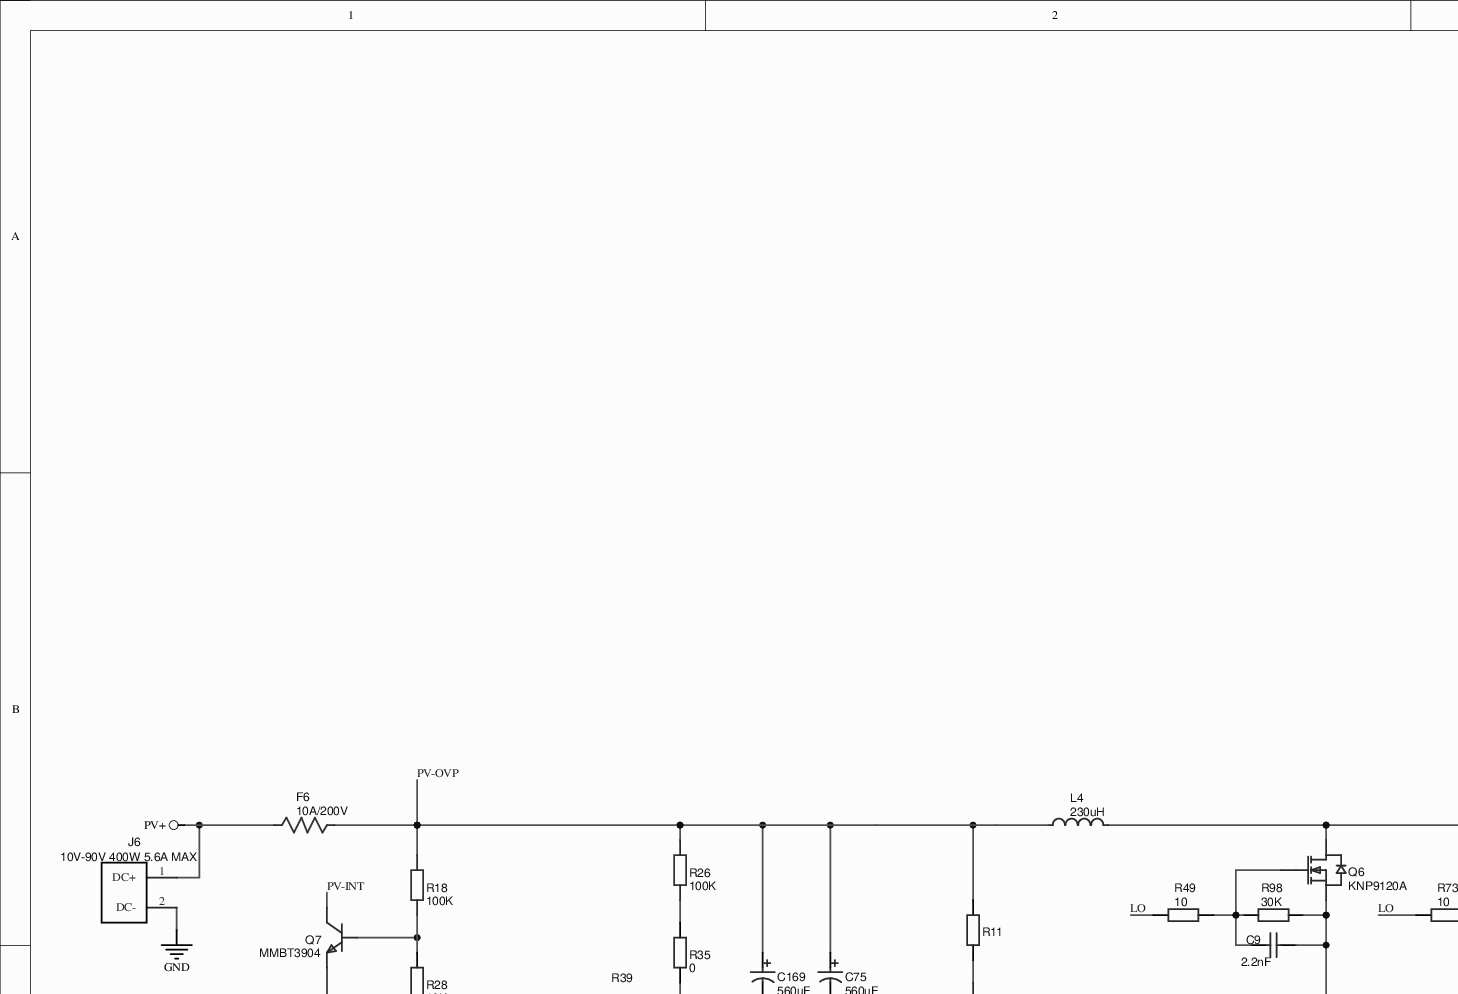
[diagram p0: MISC89356-2.schdoc, top left]
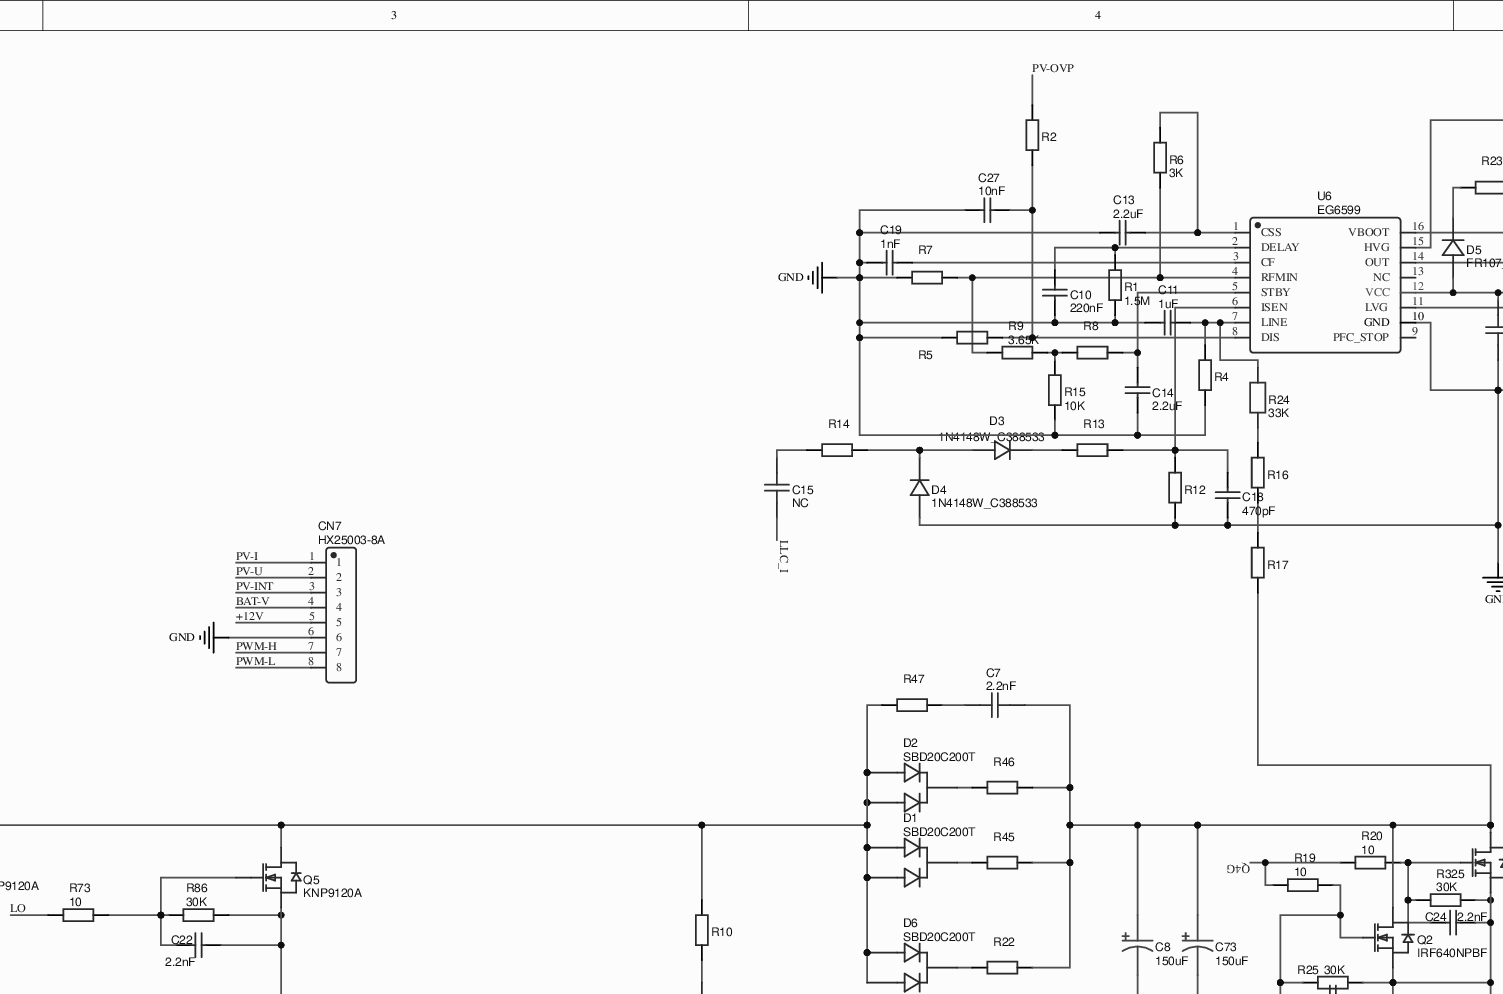
[diagram p1: MISC89356-2.schdoc, top middle]
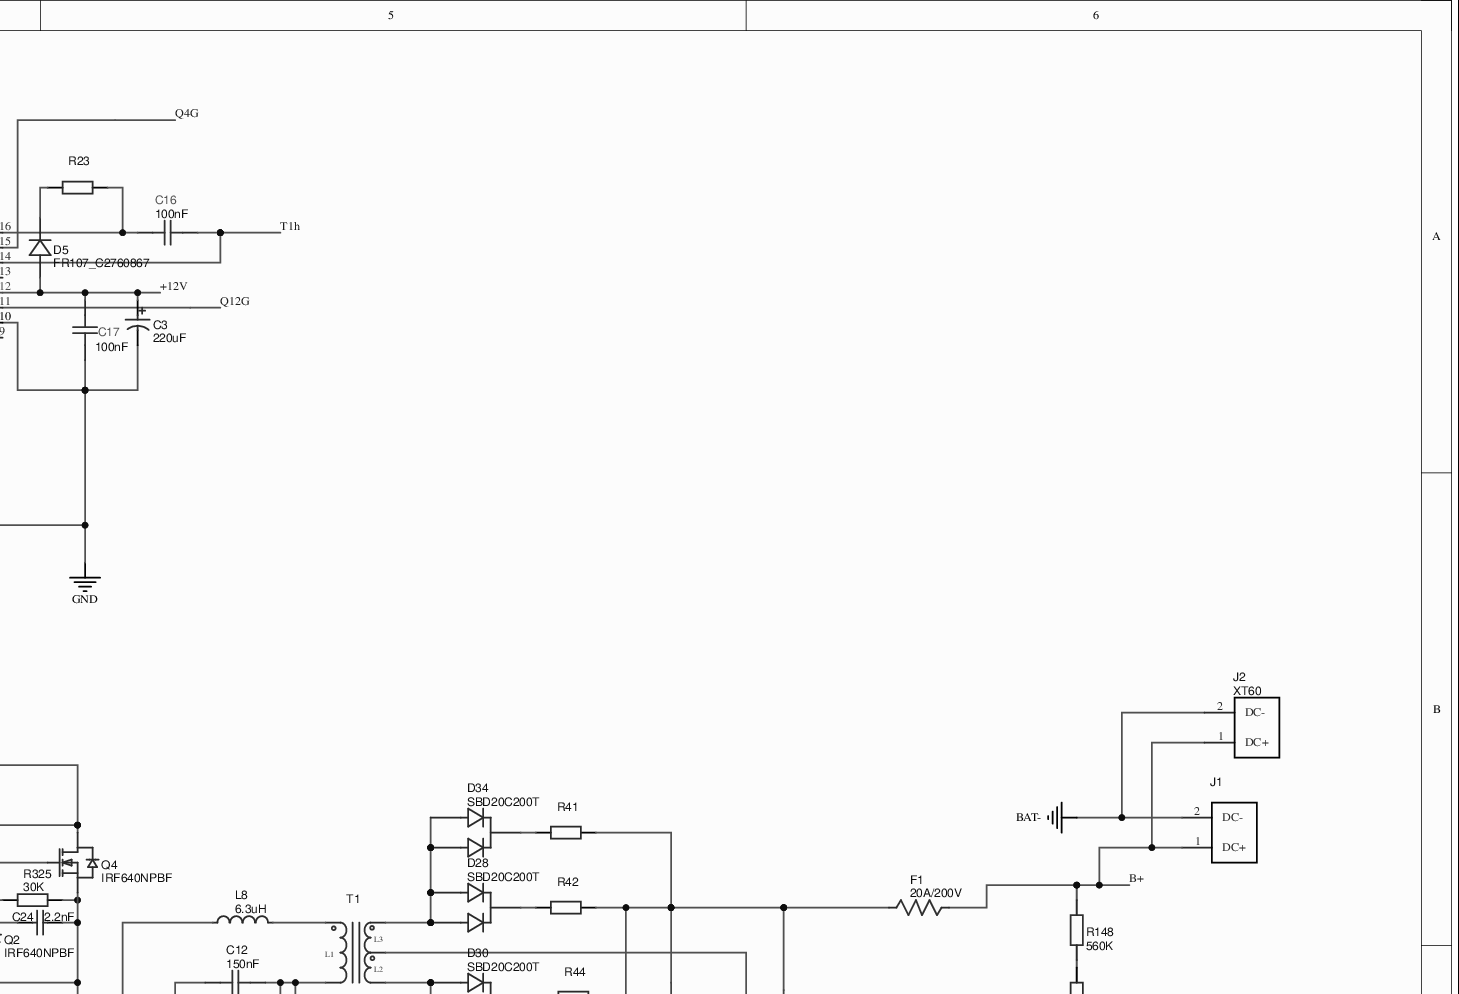
[diagram p2: MISC89356-2.schdoc, top right]
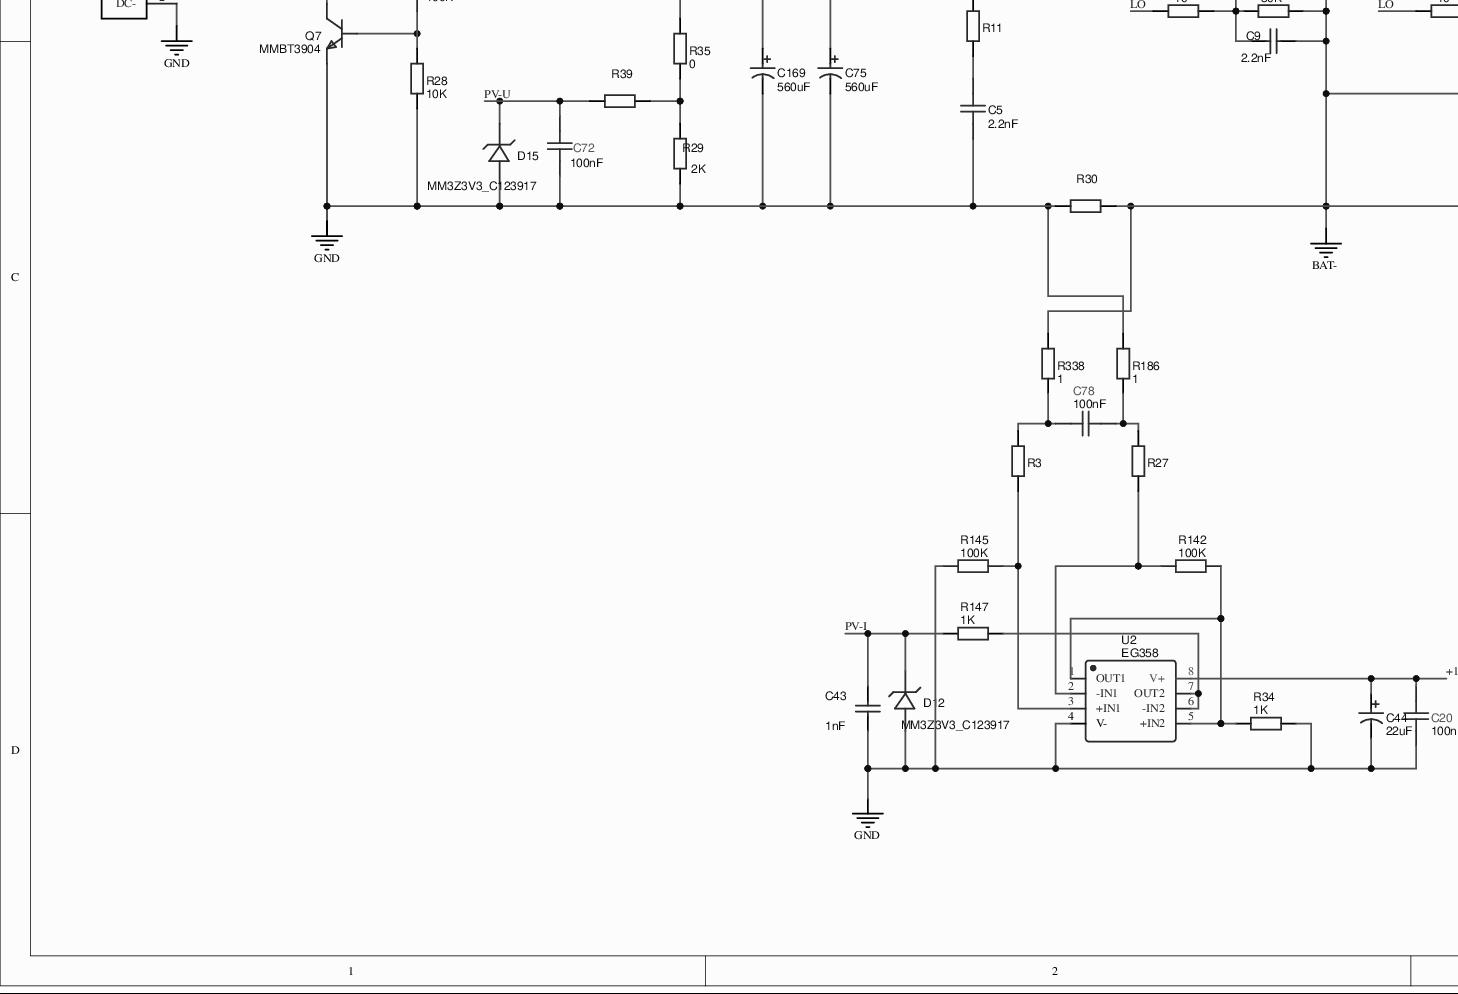
[diagram p3: MISC89356-2.schdoc, bottom left]
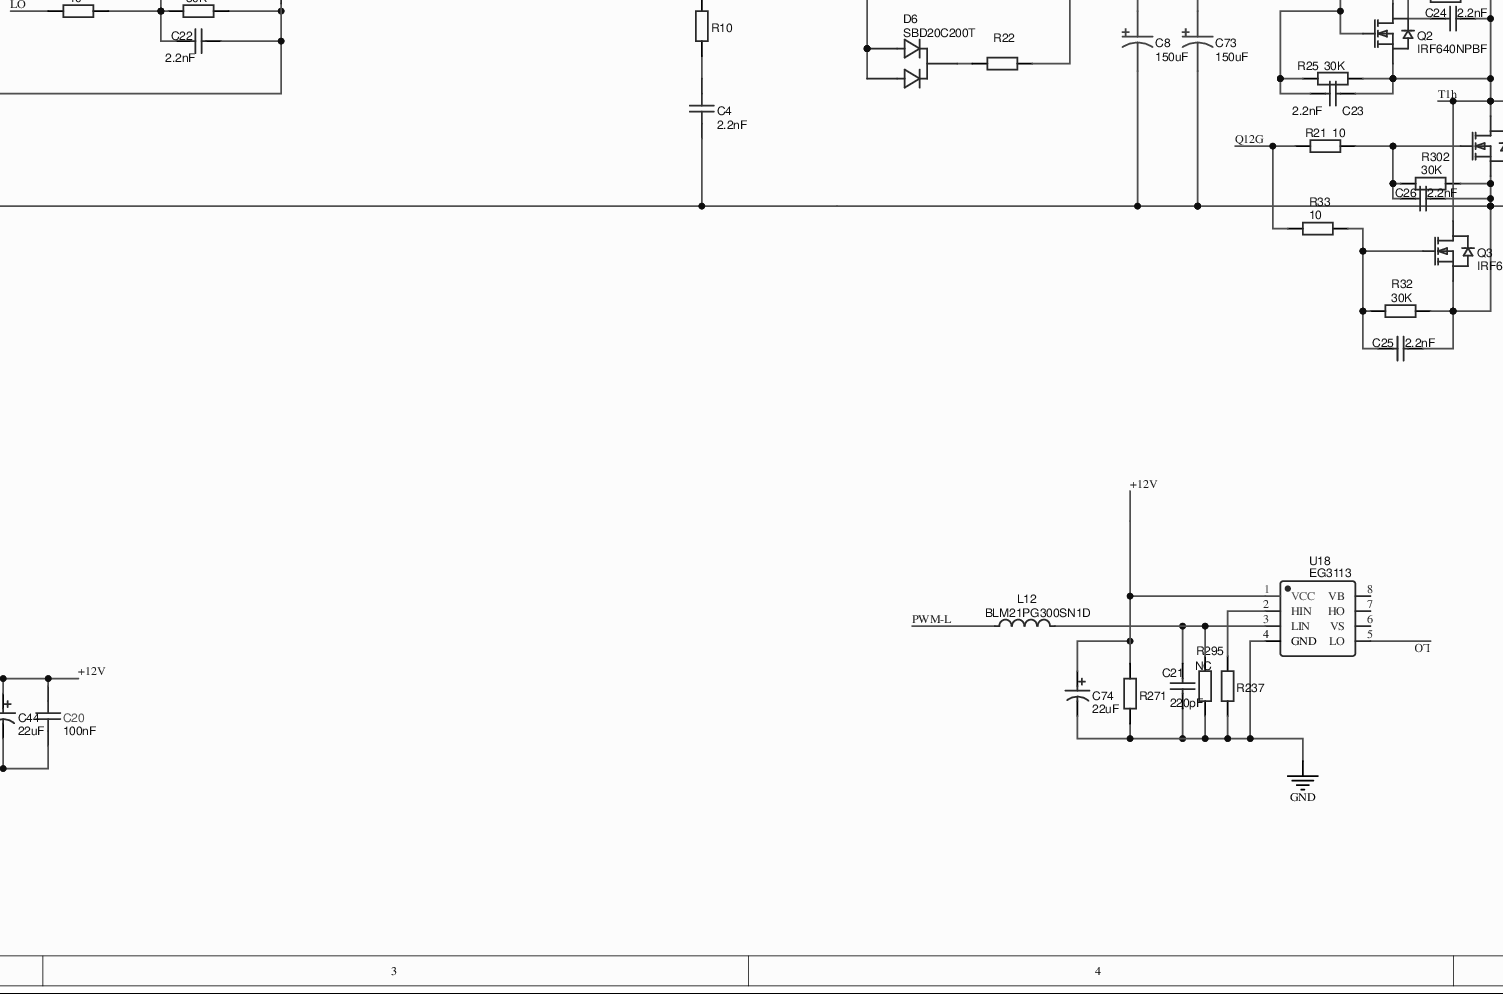
[diagram p4: MISC89356-2.schdoc, bottom middle]
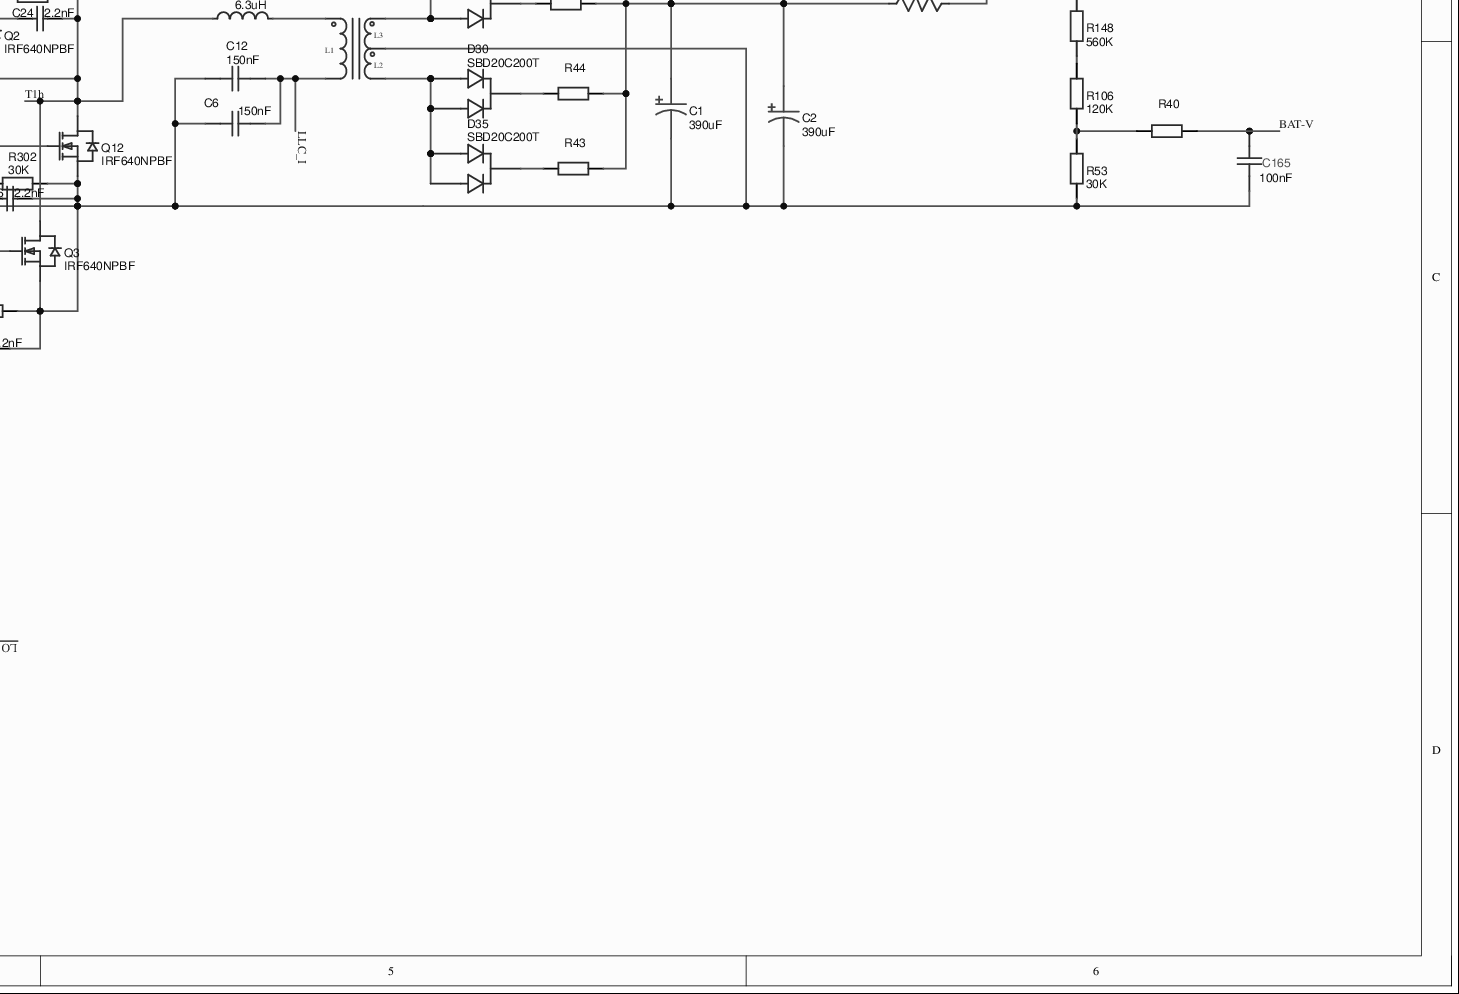
[diagram p5: MISC89356-2.schdoc, bottom right]
# Altium project MISC89356-11.PrjPCB
1 sheet, 128 parts. Net scope: global (net labels, ports and power ports of the same name join across sheets).
Board file: MISC89356.PcbDoc

## Sheet MISC89356-2.schdoc
size 715 x 319 mm

### Parts
C1  390uF  [CAP-TH_BD10.0-P5.00-D1.0-FD]
C2  390uF  [CAP-TH_BD10.0-P5.00-D1.0-FD]
C3  220uF  [CAP-TH_BD6.3-P2.50-D1.0-FD]
C4  2.2nF  [C1206]
C5  2.2nF  [C1206]
C6  150nF  [CAP-TH_L17.0-W6.5-P15.00-D1.2]
C7  2.2nF  [C1206]
C8  150uF  [CAP-TH_BD12.5-P5.00-D0.6-FD]
C9  2.2nF  [C0603]
C10  220nF  [C0603]
C11  1uF  [C0603]
C12  150nF  [CAP-TH_L17.0-W6.5-P15.00-D1.2]
C13  2.2uF  [C0603]
C14  2.2uF  [C0603]
C15  NC  [C1206]
C16  100nF  [C0603]
C17  100nF  [C0603]
C18  470pF  [C0603]
C19  1nF  [C0603]
C20  100nF  [C0603]
C21  220pF  [C0603]
C22  2.2nF  [C0603]
C23  2.2nF  [C0603]
C24  2.2nF  [C0603]
C25  2.2nF  [C0603]
C26  2.2nF  [C0603]
C27  10nF  [C1206]
C43  1nF  [C0603]
C44  22uF  [CAP-TH_BD5.0-P2.00-D0.8-FD]
C72  100nF  [C0603]
C73  150uF  [CAP-TH_BD12.5-P5.00-D0.6-FD]
C74  22uF  [CAP-TH_BD5.0-P2.00-D0.8-FD]
C75  560uF  [CAP-TH_BD16.0-P7.50-D1.2-FD]
C78  100nF  [C0603]
C165  100nF  [C0603]
C169  560uF  [CAP-TH_BD16.0-P7.50-D1.2-FD]
CN7  HX25003-8A  [CONN-TH_8P-P2.50_HX25003-8A]
D1  SBD20C200T  [TO-220-3_L10.0-W4.5-P2.54-L]
D2  SBD20C200T  [TO-220-3_L10.0-W4.5-P2.54-L]
D3  1N4148W_C388533  [SOD-123_L2.8-W1.8-LS3.7-RD]
D4  1N4148W_C388533  [SOD-123_L2.8-W1.8-LS3.7-RD]
D5  FR107_C2760867  [SOD-123FL_L2.7-W1.8-LS3.8-RD]
D6  SBD20C200T  [TO-220-3_L10.0-W4.5-P2.54-L]
D12  MM3Z3V3_C123917  [SOD-323_L1.8-W1.3-LS2.5-RD]
D15  MM3Z3V3_C123917  [SOD-323_L1.8-W1.3-LS2.5-RD]
D28  SBD20C200T  [TO-220-3_L10.0-W4.5-P2.54-L-N]
D30  SBD20C200T  [TO-220-3_L10.0-W4.5-P2.54-L-N]
D34  SBD20C200T  [TO-220-3_L10.0-W4.5-P2.54-L-N]
D35  SBD20C200T  [TO-220-3_L10.0-W4.5-P2.54-L-N]
F1  20A/200V  [FUSE-SMD_L6.1-W2.5]
F6  10A/200V  [FUSE-SMD_L6.1-W2.5]
J1  (no value)  [XT90N]
J2  XT60  [CONN-TH_XT60UPB-F]
J6  10V-90V 400W 5.6A MAX  [XT90]
L4  230uH  [IND-TH_CS343090*2-W231K]
L8  6.3uH  [PQ2620-N]
L12  BLM21PG300SN1D  [L0805]
Q2  IRF640NPBF  [TO-220-3_L10.0-W4.5-P2.54-L-N]
Q3  IRF640NPBF  [TO-220-3_L10.0-W4.5-P2.54-L-N]
Q4  IRF640NPBF  [TO-220-3_L10.0-W4.5-P2.54-L-N]
Q5  KNP9120A  [TO-220-3_L10.0-W4.5-P2.54-L]
Q6  KNP9120A  [TO-220-3_L10.0-W4.5-P2.54-L]
Q7  MMBT3904  [SOT-23-3_L2.9-W1.3-P1.90-LS2.4-BR]
Q12  IRF640NPBF  [TO-220-3_L10.0-W4.5-P2.54-L-N]
R1  1.5M  [R0603]
R2  (no value)  [R0805]
R3  (no value)  [R0603]
R4  (no value)  [R0603]
R5  (no value)  [R0805]
R6  3K  [R0603]
R7  (no value)  [R0603]
R8  (no value)  [R0603]
R9  3.65K  [R0603]
R10  (no value)  [R1206]
R11  (no value)  [R1206]
R12  (no value)  [R0603]
R13  (no value)  [R0603]
R14  (no value)  [R0603]
R15  10K  [R1206]
R16  (no value)  [R1206]
R17  (no value)  [R1206]
R18  100K  [R0805]
R19  10  [R1206]
R20  10  [R1206]
R21  10  [R1206]
R22  (no value)  [R2512]
R23  (no value)  [R0805]
R24  33K  [R1206]
R25  30K  [R0603]
R26  100K  [R0805]
R27  (no value)  [R0603]
R28  10K  [R1206]
R29  2K  [R0603]
R30  (no value)  [R2512]
R32  30K  [R0603]
R33  10  [R1206]
R34  1K  [R0603]
R35  0  [R0805]
R39  (no value)  [R0603]
R40  (no value)  [R0603]
R41  (no value)  [R2512]
R42  (no value)  [R2512]
R43  (no value)  [R2512]
R44  (no value)  [R2512]
R45  (no value)  [R2512]
R46  (no value)  [R2512]
R47  (no value)  [R1206]
R49  10  [R1206]
R53  30K  [R0603]
R73  10  [R1206]
R86  30K  [R0603]
R98  30K  [R0603]
R106  120K  [R0603]
R142  100K  [R0805]
R145  100K  [R0805]
R147  1K  [R0603]
R148  560K  [R0603]
R186  1  [R0603]
R237  (no value)  [R0603]
R271  (no value)  [R0603]
R295  NC  [R0603]
R302  30K  [R0603]
R325  30K  [R0603]
R338  1  [R0603]
T1  (no value)  [PQ3230 3:2:2-N]
U2  EG358  [SOIC-8_L5.0-W4.0-P1.27-LS6.0-BL]
U6  EG6599  [SO-16_L10.0-W4.0-P1.27-LS6.2-BL]
U18  EG3113  [SOP-8_L4.9-W3.9-P1.27-LS6.0-BL]

### Nets
BAT-: C1.2 C2.2 C4.2 C6.2 C8.2 C9.2 C12.2 C22.2 C25.2 C26.2 C73.2 C165.1 J1.2(DC-) J2.2(DC-) Q3.3(S) Q5.3(S) Q6.3(S) Q12.3(S) R30.2 R32.2 R53.1 R86.1 R98.1 R302.2 R338.2 T1.9
GND: C3.2 C5.2 C10.1 C11.2 C13.1 C14.1 C17.1 C18.1 C19.2 C20.2 C21.1 C27.1 C43.1 C44.2 C72.1 C74.2 C75.2 C169.2 CN7.6 D4.2(A) D12.2(A) D15.2(A) J6.2(DC-) Q7.2(E) R1.1 R4.1 R5.1 R7.2 R12.1 R15.2 R28.2 R29.2 R30.1 R34.2 R145.2 R186.2 R237.1 R271.1 R295.2 U2.4(V-) U6.10(GND) U18.4(GND)
PV+: F6.1 J6.1(DC+)
+12V: C3.1 C17.2 C20.1 C44.1 C74.1 CN7.5 D5.2(A) R271.2 U2.8(V+) U6.12(VCC) U18.1(VCC)
B+: F1.2 J1.1(DC+) J2.1(DC+) R148.2
BAT-V: C165.2 CN7.4 R40.1
LLC_I: C6.1 C12.1 C15.1 T1.3
LO: R49.1 R73.1 U18.5(LO)
PV-I: C43.2 CN7.1 D12.1(K) R147.2
PV-INT: CN7.3 Q7.3(C)
PV-OVP: C75.1 C169.1 F6.2 L4.1 R2.2 R11.1 R18.2 R26.2
PV-U: C72.2 CN7.2 D15.1(K) R39.2
PWM-H: CN7.7
PWM-L: CN7.8 L12.1
Q4G: R19.1 R20.1 U6.15(HVG)
Q12G: R21.1 R33.1 U6.11(LVG)
T1h: C16.1 C23.2 C24.2 L8.3 Q2.3(S) Q3.2(D) Q4.3(S) Q12.2(D) R25.2 R325.2 U6.14(OUT)
NetC1_1: C1.1 C2.1 F1.1 R41.2 R42.2 R43.2 R44.2
NetC4_1: C4.1 R10.2
NetC5_1: C5.1 R11.2
NetC7_1: C7.1 R47.2
NetC7_2: C7.2 C8.1 C73.1 Q2.2(D) Q4.2(D) R17.1 R22.2 R45.2 R46.2
NetC9_1: C9.1 Q6.1(G) R49.2 R98.2
NetC10_2: C10.2 R1.2 U6.2(DELAY)
NetC11_1: C11.1 R4.2 R24.2 U6.7(LINE)
NetC13_2: C13.2 R6.2 U6.1(CSS)
NetC14_2: C14.2 R8.2 U6.5(STBY)
NetC15_2: C15.2 R14.1
NetC16_2: C16.2 R23.1 U6.16(VBOOT)
NetC18_2: C18.2 R12.2 R13.2 U6.6(ISEN)
NetC19_1: C19.1 U6.3(CF)
NetC21_2: C21.2 L12.2 R295.1 U18.3(LIN)
NetC22_1: C22.1 Q5.1(G) R73.2 R86.2
NetC23_1: C23.1 Q2.1(G) R19.2 R25.1
NetC24_1: C24.1 Q4.1(G) R20.2 R325.1
NetC25_1: C25.1 Q3.1(G) R32.1 R33.2
NetC26_1: C26.1 Q12.1(G) R21.2 R302.1
NetC27_2: C27.2 R2.1 R5.2 U6.8(DIS)
NetC78_1: C78.1 R27.2 R186.1
NetC78_2: C78.2 R3.2 R338.1
NetD1_1: D1.1 D1.3 D2.1 D2.3 D6.1 D6.3 L4.2 Q5.2(D) Q6.2(D) R10.1 R47.1
NetD1_2: D1.2 R45.1
NetD2_2: D2.2 R46.1
NetD3_1: D3.1(C) R13.1
NetD3_2: D3.2(A) D4.1(C) R14.2
NetD5_1: D5.1(K) R23.2
NetD6_2: D6.2 R22.1
NetD28_1: D28.1 D28.3 D34.1 D34.3 T1.8
NetD28_2: D28.2 R42.1
NetD30_1: D30.1 D30.3 D35.1 D35.3 T1.10
NetD30_2: D30.2 R44.1
NetD34_2: D34.2 R41.1
NetD35_2: D35.2 R43.1
NetL8_4: L8.4 T1.4
NetQ7_1: Q7.1(B) R18.1 R28.1
NetR3_1: R3.1 R145.1 U2.3(+IN1)
NetR6_1: R6.1 R7.1 R9.1 U6.4(RFMIN)
NetR8_1: R8.1 R9.2 R15.1
NetR16_1: R16.1 R17.2
NetR16_2: R16.2 R24.1
NetR26_1: R26.1 R35.2
NetR27_1: R27.1 R142.2 U2.2(-IN1)
NetR29_1: R29.1 R35.1 R39.1
NetR34_1: R34.1 R142.1 U2.1(OUT1) U2.5(+IN2)
NetR40_2: R40.2 R53.2 R106.1
NetR106_2: R106.2 R148.1
NetR147_1: R147.1 U2.6(-IN2) U2.7(OUT2)
NetR237_2: R237.2 U18.2(HIN)

Not connected (* = marked no-connect by the designer): U6 9(PFC_STOP) 13(NC); U18 6(VS) 7(HO) 8(VB)

### Library data of the parts
C1 C2 = 390uF: BOM_Manufacturer: Ymin; BOM_Manufacturer Part: LKME2001J391MF; nameAlias: Capacitance; Contributor: LCSC; BOM_Supplier: LCSC; BOM_Supplier Part: C442948; BOM_JLCPCB Part Class: Extended Part; spicePre: C; spiceSymbolName: LKME2001J391MF
C3 = 220uF: BOM_Manufacturer: ValuePro; BOM_Manufacturer Part: 220uF 16V 6.3*11; nameAlias: Capacitance; BOM_Supplier: LCSC; BOM_Supplier Part: C43349; BOM_JLCPCB Part Class: Extended Part; spicePre: C; spiceSymbolName: 220uF 16V 6.3*11
C4 C5 C7 = 2.2nF: BOM_Manufacturer: Johanson Dielectrics; BOM_Manufacturer Part: 202R18W222KV4E; nameAlias: Capacitance; Contributor: LCSC; BOM_Supplier: LCSC; BOM_Supplier Part: C173213; BOM_JLCPCB Part Class: Extended Part; spicePre: C; spiceSymbolName: 202R18W222KV4E
C6 C12 = 150nF: BOM_Manufacturer: KYET; BOM_Manufacturer Part: KP154J2J1501; nameAlias: Capacitance; Contributor: LCSC; BOM_Supplier: LCSC; BOM_Supplier Part: C390138; BOM_JLCPCB Part Class: Extended Part; spicePre: C; spiceSymbolName: KP154J2J1501
C8 C73 = 150uF: BOM_Manufacturer: Ymin; BOM_Manufacturer Part: LKML2502C151MF; nameAlias: Capacitance; Contributor: LCSC; BOM_Supplier: LCSC; BOM_Supplier Part: C443216; BOM_JLCPCB Part Class: Extended Part; spicePre: C; spiceSymbolName: LKML2502C151MF
C9 C22-C26 = 2.2nF: BOM_Manufacturer: YAGEO; BOM_Manufacturer Part: CC0603KRX7R9BB222; nameAlias: Capacitance; BOM_Supplier: LCSC; BOM_Supplier Part: C107082; BOM_JLCPCB Part Class: Extended Part; spicePre: C; spiceSymbolName: CC0603KRX7R9BB222
C10 = 220nF: BOM_Manufacturer Part: CL10B224KA8NNNC; BOM_Manufacturer: SAMSUNG; nameAlias: Capacitance; BOM_Supplier: LCSC; BOM_Supplier Part: C21120; BOM_JLCPCB Part Class: Basic Part; spicePre: C; spiceSymbolName: CL10B224KA8NNNC
C11 = 1uF: BOM_Manufacturer Part: CL10A105KB8NNNC; BOM_Manufacturer: SAMSUNG; nameAlias: Capacitance; BOM_Supplier: LCSC; BOM_Supplier Part: C15849; BOM_JLCPCB Part Class: Basic Part; spicePre: C; spiceSymbolName: CL10A105KB8NNNC
C13 C14 = 2.2uF: BOM_Manufacturer Part: CL10A225KO8NNNC; BOM_Manufacturer: SAMSUNG; nameAlias: Capacitance; BOM_Supplier: LCSC; BOM_Supplier Part: C23630; BOM_JLCPCB Part Class: Basic Part; spicePre: C; spiceSymbolName: CL10A225KO8NNNC
C15 = NC: BOM_Manufacturer: Guangdong Fenghua Advanced Tech; BOM_Manufacturer Part: 1206CG220J102NT; nameAlias: Capacitance; Contributor: LCSC; BOM_Supplier: LCSC; BOM_Supplier Part: C313096; BOM_JLCPCB Part Class: Extended Part; spicePre: C; spiceSymbolName: 1206CG220J102NT
C16 C17 C20 C72 C78 C165 = 100nF: BOM_Manufacturer: SAMSUNG; BOM_Manufacturer Part: CL10B104KC8NNNC; nameAlias: Capacitance; BOM_Supplier: LCSC; BOM_Supplier Part: C15725; BOM_JLCPCB Part Class: Extended Part; spicePre: C; spiceSymbolName: CL10B104KC8NNNC
C18 = 470pF: BOM_Manufacturer: FH; BOM_Manufacturer Part: 0603B471K500NT; nameAlias: Capacitance; BOM_Supplier: LCSC; BOM_Supplier Part: C1620; BOM_JLCPCB Part Class: Basic Part; spicePre: C; spiceSymbolName: 0603B471K500NT
C19 = 1nF: BOM_Manufacturer: SAMSUNG; BOM_Manufacturer Part: CL10B102KB8NNNC; nameAlias: Capacitance; Contributor: LCSC; BOM_Supplier: LCSC; BOM_Supplier Part: C1588; BOM_JLCPCB Part Class: Extended Part; spicePre: C; spiceSymbolName: CL10B102KC8NNNC
C21 = 220pF: BOM_Manufacturer: YAGEO; BOM_Manufacturer Part: CC0603KRX7R9BB221; nameAlias: Capacitance; BOM_Supplier: LCSC; BOM_Supplier Part: C107081; BOM_JLCPCB Part Class: Extended Part; spicePre: C; spiceSymbolName: CC0603KRX7R9BB221
C27 = 10nF: BOM_Manufacturer: FH; BOM_Manufacturer Part: 1206B103K102NT; nameAlias: Capacitance; BOM_Supplier: LCSC; BOM_Supplier Part: C9194; BOM_JLCPCB Part Class: Extended Part; spicePre: C; spiceSymbolName: 1206B103K102NT
C43 = 1nF: BOM_Manufacturer Part: CL10B102KB8NNNC; BOM_Manufacturer: SAMSUNG; nameAlias: Capacitance; BOM_Supplier: LCSC; BOM_Supplier Part: C1588; BOM_JLCPCB Part Class: Basic Part; spicePre: C; spiceSymbolName: CL10B102KB8NNNC
C44 C74 = 22uF: BOM_Manufacturer: ValuePro; BOM_Manufacturer Part: 22uF 50V 5*11; nameAlias: Capacitance; BOM_Supplier: LCSC; BOM_Supplier Part: C43346; BOM_JLCPCB Part Class: Extended Part; spicePre: C; spiceSymbolName: 22uF 50V 5*11
C75 C169 = 560uF: BOM_Manufacturer: Rubycon; BOM_Manufacturer Part: 35YXJ2200M16X25; nameAlias: Capacitance; BOM_Supplier: LCSC; BOM_Supplier Part: C95096; BOM_JLCPCB Part Class: Extended Part; spicePre: C; spiceSymbolName: 35YXJ2200M16X25
CN7 = HX25003-8A: BOM_Manufacturer: HX(Zhejiang Yueqing Hongxing Elec); Contributor: LCSC; BOM_Supplier: LCSC; BOM_Supplier Part: C442305; BOM_Manufacturer Part: HX25003-8A; BOM_JLCPCB Part Class: Extended Part; spicePre: C; spiceSymbolName: HX25003-8A
D1 D2 D6 D28 D30 D34 D35 = SBD20C200T: BOM_Manufacturer: PANJIT; BOM_Manufacturer Part: SBT40100VCT; Contributor: LCSC; BOM_Supplier Part: C142331; BOM_Supplier: LCSC; BOM_JLCPCB Part Class: Extended Part; spicePre: D; spiceSymbolName: SBT40100VCT
D3 D4 = 1N4148W_C388533: BOM_Manufacturer: Yangzhou Yangjie Elec Tech; Contributor: LCSC; BOM_Supplier: LCSC; BOM_Supplier Part: C388533; BOM_Manufacturer Part: 1N4148W; BOM_JLCPCB Part Class: Extended Part; spicePre: D; spiceSymbolName: 1N4148W_C388533
D5 = FR107_C2760867: BOM_Manufacturer Part: FR107; Contributor: LCSC; BOM_Supplier: LCSC; BOM_Supplier Part: C2760867; BOM_JLCPCB Part Class: Extended Part; spicePre: D; spiceSymbolName: FR107_C2760867
D12 D15 = MM3Z3V3_C123917: BOM_Manufacturer: Shandong Jingdao Microelectronics; Contributor: LCSC; BOM_Supplier: LCSC; BOM_Supplier Part: C123917; BOM_Manufacturer Part: MM3Z3V3; BOM_JLCPCB Part Class: Extended Part; spicePre: D; spiceSymbolName: MM3Z3V3_C123917
F1 = 20A/200V: Contributor: LCEDA_Lib; spicePre: R; spiceSymbolName: R_1206_US
F6 = 10A/200V: Contributor: LCEDA_Lib; spicePre: R; spiceSymbolName: R_1206_US
J1 = (no symbol name): BOM_Manufacturer: ReliaPro; BOM_Manufacturer Part: TJC1-2A; BOM_Supplier: LCSC; BOM_Supplier Part: C29632; spicePre: J; spiceSymbolName: TJC1-2A
J2 = XT60: BOM_Manufacturer: ReliaPro; BOM_Manufacturer Part: TJC1-2A; BOM_Supplier: LCSC; BOM_Supplier Part: C29632; spicePre: J; spiceSymbolName: TJC1-2A
J6 = 10V-90V 400W 5.6A MAX: BOM_Manufacturer: ReliaPro; BOM_Manufacturer Part: TJC1-2A; BOM_Supplier: LCSC; BOM_Supplier Part: C29632; spicePre: J; spiceSymbolName: TJC1-2A
L4 = 230uH: nameAlias: Value(H); Contributor: LCEDA_Lib; spicePre: L; spiceSymbolName: L0402_US
L8 = 6.3uH: nameAlias: Value(H); Contributor: LCEDA_Lib; spicePre: L; spiceSymbolName: L0402_US
L12 = BLM21PG300SN1D: BOM_Manufacturer: MuRata; nameAlias: Value(H); BOM_Supplier: LCSC; BOM_Manufacturer Part: BLM21PG300SN1D; BOM_Supplier Part: C16903; BOM_JLCPCB Part Class: Extended Part; spicePre: L; spiceSymbolName: BLM21PG300SN1D
Q2-Q4 Q12 = IRF640NPBF: BOM_Manufacturer: Infineon; BOM_Supplier: LCSC; BOM_Manufacturer Part: IRF640NPBF; BOM_Supplier Part: C2568; BOM_JLCPCB Part Class: Extended Part; spicePre: Q; spiceSymbolName: IRF640NPBF
Q5 Q6 = KNP9120A: BOM_Manufacturer: KIA; BOM_Supplier: LCSC; BOM_Manufacturer Part: KNP9120A; BOM_Supplier Part: C135565; BOM_JLCPCB Part Class: Extended Part; spicePre: Q; spiceSymbolName: KNP9120A
Q7 = MMBT3904: Contributor: LCSC; BOM_Supplier: LCSC; BOM_Supplier Part: C2688228; BOM_Manufacturer Part: MMBT3904; BOM_JLCPCB Part Class: Extended Part; spicePre: Q; spiceSymbolName: MMBT3904
R1 = 1.5M: BOM_Manufacturer: YAGEO; BOM_Manufacturer Part: RC0603FR-071M5L; nameAlias: Resistance (Ohms); BOM_Supplier: LCSC; BOM_Supplier Part: C137773; BOM_JLCPCB Part Class: Extended Part; spicePre: R; spiceSymbolName: RC0603FR-071M5L
R2 = (no symbol name): BOM_Manufacturer: UniOhm; BOM_Manufacturer Part: 0805W8F4753T5E; nameAlias: Resistance; Resistance (Ohms): 475K; BOM_Supplier: LCSC; BOM_Supplier Part: C17711; BOM_JLCPCB Part Class: Extended Part; spicePre: R; spiceSymbolName: 0805W8F4753T5E
R3 R12 R27 = (no symbol name): BOM_Manufacturer: UniOhm; BOM_Manufacturer Part: 0603WAF1501T5E; nameAlias: Resistance; Resistance (Ohms): 1.5K; BOM_Supplier: LCSC; BOM_Supplier Part: C22843; BOM_JLCPCB Part Class: Basic Part; spicePre: R; spiceSymbolName: 0603WAF1501T5E
R4 R14 R271 = (no symbol name): BOM_Manufacturer: UniOhm; BOM_Manufacturer Part: 0603WAF1002T5E; nameAlias: Resistance; Resistance (Ohms): 10K; BOM_Supplier: LCSC; BOM_Supplier Part: C25804; BOM_JLCPCB Part Class: Basic Part; spicePre: R; spiceSymbolName: 0603WAF1002T5E
R5 = (no symbol name): BOM_Manufacturer: UniOhm; BOM_Manufacturer Part: 0805W8F9101T5E; nameAlias: Resistance; Resistance (Ohms): 9.1K; BOM_Supplier: LCSC; BOM_Supplier Part: C17855; BOM_JLCPCB Part Class: Basic Part; spicePre: R; spiceSymbolName: 0805W8F9101T5E
R6 = 3K: BOM_Manufacturer: YAGEO; BOM_Manufacturer Part: RC0603FR-073KL; nameAlias: Resistance (Ohms); BOM_Supplier: LCSC; BOM_Supplier Part: C126358; BOM_JLCPCB Part Class: Extended Part; spicePre: R; spiceSymbolName: RC0603FR-073KL
R7 = (no symbol name): BOM_Manufacturer: UniOhm; BOM_Manufacturer Part: 0603WAF4701T5E; nameAlias: Resistance; Resistance (Ohms): 4.7K; BOM_Supplier: LCSC; BOM_Supplier Part: C23162; BOM_JLCPCB Part Class: Basic Part; spicePre: R; spiceSymbolName: 0603WAF4701T5E
R8 R237 = (no symbol name): BOM_Manufacturer: UniOhm; BOM_Manufacturer Part: 0603WAF0000T5E; nameAlias: Resistance; Resistance (Ohms): 0; BOM_Supplier: LCSC; BOM_Supplier Part: C21189; BOM_JLCPCB Part Class: Basic Part; spicePre: R; spiceSymbolName: 0603WAF0000T5E
R9 = 3.65K: BOM_Manufacturer: YAGEO; BOM_Manufacturer Part: RC0603FR-073K65L; nameAlias: Resistance (Ohms); BOM_Supplier: LCSC; BOM_Supplier Part: C137730; BOM_JLCPCB Part Class: Extended Part; spicePre: R; spiceSymbolName: RC0603FR-073K65L
R10 R11 R47 = (no symbol name): BOM_Manufacturer: UniOhm; BOM_Manufacturer Part: 1206W4F100KT5E; nameAlias: Resistance; Resistance (Ohms): 1; BOM_Supplier: LCSC; BOM_Supplier Part: C17928; BOM_JLCPCB Part Class: Basic Part; spicePre: R; spiceSymbolName: 1206W4F100KT5E
R13 = (no symbol name): BOM_Manufacturer: UniOhm; BOM_Manufacturer Part: 0603WAF510JT5E; nameAlias: Resistance; Resistance (Ohms): 51; BOM_Supplier: LCSC; BOM_Supplier Part: C23197; BOM_JLCPCB Part Class: Basic Part; spicePre: R; spiceSymbolName: 0603WAF510JT5E
R15 R28 = 10K: BOM_Manufacturer: UniOhm; BOM_Manufacturer Part: 1206W4F1002T5E; nameAlias: Resistance (Ohms); BOM_Supplier: LCSC; BOM_Supplier Part: C17902; BOM_JLCPCB Part Class: Basic Part; spicePre: R; spiceSymbolName: 1206W4F1002T5E
R16 R17 = (no symbol name): BOM_Manufacturer: UniOhm; BOM_Manufacturer Part: 1206W4F3003T5E; nameAlias: Resistance; Resistance (Ohms): 300K; BOM_Supplier: LCSC; BOM_Supplier Part: C17884; BOM_JLCPCB Part Class: Extended Part; spicePre: R; spiceSymbolName: 1206W4F3003T5E
R18 R26 R142 R145 = 100K: BOM_Manufacturer: YAGEO; BOM_Manufacturer Part: RC0805JR-07100KL; nameAlias: Resistance (Ohms); Contributor: LCSC; BOM_Supplier: LCSC; BOM_Supplier Part: C100049; BOM_JLCPCB Part Class: Extended Part; spicePre: R; spiceSymbolName: RC0805JR-07100KL
R19-R21 R33 R49 R73 = 10: BOM_Manufacturer: LIZ; BOM_Manufacturer Part: CR1206J40100G; nameAlias: Resistance (Ohms); BOM_Supplier: LCSC; BOM_Supplier Part: C102266; BOM_JLCPCB Part Class: Extended Part; spicePre: R; spiceSymbolName: CR1206J40100G
R22 R41-R46 = (no symbol name): BOM_Manufacturer: RALEC; BOM_Manufacturer Part: RTT25R100FTE; nameAlias: Resistance; Resistance (Ohms): 0.1; BOM_Supplier: LCSC; BOM_Supplier Part: C105145; BOM_JLCPCB Part Class: Extended Part; spicePre: R; spiceSymbolName: RTT25R100FTE
R23 = (no symbol name): BOM_Manufacturer: UniOhm; BOM_Manufacturer Part: 0805W8F220KT5E; nameAlias: Resistance; Resistance (Ohms): 2.2; BOM_Supplier: LCSC; BOM_Supplier Part: C17521; BOM_JLCPCB Part Class: Basic Part; spicePre: R; spiceSymbolName: 0805W8F220KT5E
R24 = 33K: BOM_Manufacturer: YAGEO; BOM_Manufacturer Part: AC1206JR-0733KL; nameAlias: Resistance (Ohms); Contributor: LCSC; BOM_Supplier: LCSC; BOM_Supplier Part: C229931; BOM_JLCPCB Part Class: Extended Part; spicePre: R; spiceSymbolName: AC1206JR-0733KL
R25 R32 R53 R86 R98 R302 R325 = 30K: BOM_Manufacturer: UniOhm; BOM_Manufacturer Part: 0805W8F3002T5E; nameAlias: Resistance (Ohms); BOM_Supplier: LCSC; BOM_Supplier Part: C17621; BOM_JLCPCB Part Class: Basic Part; spicePre: R; spiceSymbolName: 0805W8F3002T5E
R29 = 2K: BOM_Manufacturer: UniOhm; BOM_Manufacturer Part: 0603WAF2001T5E; nameAlias: Resistance (Ohms); BOM_Supplier: LCSC; BOM_Supplier Part: C22975; BOM_JLCPCB Part Class: Basic Part; spicePre: R; spiceSymbolName: 0603WAF2001T5E
R30 = (no symbol name): BOM_Manufacturer: PSA; BOM_Manufacturer Part: FMF25FPHR005-LHL; nameAlias: Resistance; Resistance (Ohms): 0.005; BOM_Supplier: LCSC; BOM_Supplier Part: C105361; BOM_JLCPCB Part Class: Extended Part; spicePre: R; spiceSymbolName: FMF25FPHR005-LHL
R34 R147 = 1K: BOM_Manufacturer: FH; BOM_Manufacturer Part: RS-03K102JT; nameAlias: Resistance (Ohms); BOM_Supplier: LCSC; BOM_Supplier Part: C73797; spicePre: R; spiceSymbolName: RS-03K102JT
R35 = 0: BOM_Manufacturer: YAGEO; BOM_Manufacturer Part: RC0805FR-070RL; nameAlias: Resistance (Ohms); BOM_Supplier: LCSC; BOM_Supplier Part: C100045; BOM_JLCPCB Part Class: Extended Part; spicePre: R; spiceSymbolName: RC0805FR-070RL
R39 R40 = (no symbol name): BOM_Manufacturer: FH; BOM_Manufacturer Part: RS-03K102JT; nameAlias: Resistance; Resistance (Ohms): 1K; BOM_Supplier: LCSC; BOM_Supplier Part: C73797; BOM_JLCPCB Part Class: Extended Part; spicePre: R; spiceSymbolName: RS-03K102JT
R106 = 120K: BOM_Manufacturer: YAGEO; BOM_Manufacturer Part: RC0603FR-07120KL; nameAlias: Resistance (Ohms); BOM_Supplier: LCSC; BOM_Supplier Part: C114607; BOM_JLCPCB Part Class: Extended Part; spicePre: R; spiceSymbolName: RC0603FR-07120KL
R148 = 560K: BOM_Manufacturer: YAGEO; BOM_Manufacturer Part: AC0603JR-07560KL; nameAlias: Resistance (Ohms); Contributor: LCSC; BOM_Supplier: LCSC; BOM_Supplier Part: C228210; BOM_JLCPCB Part Class: Extended Part; spicePre: R; spiceSymbolName: AC0603JR-07560KL
R186 R338 = 1: BOM_Manufacturer: YAGEO; BOM_Manufacturer Part: RC0805FR-071RL; nameAlias: Resistance (Ohms); BOM_Supplier: LCSC; BOM_Supplier Part: C131397; BOM_JLCPCB Part Class: Extended Part; spicePre: R; spiceSymbolName: RC0805FR-071RL
R295 = NC: BOM_Manufacturer: FH; BOM_Manufacturer Part: RS-03K102JT; nameAlias: Resistance (Ohms); BOM_Supplier: LCSC; BOM_Supplier Part: C73797; spicePre: R; spiceSymbolName: RS-03K102JT
T1 = (no symbol name): Contributor: z123tt; spicePre: U
U2 = EG358: BOM_Manufacturer: EG; BOM_Supplier: LCSC; BOM_Manufacturer Part: EG358; BOM_Supplier Part: C111033; BOM_JLCPCB Part Class: Extended Part; spicePre: U; spiceSymbolName: EG358
U6 = EG6599: BOM_Manufacturer: EG Micro; Contributor: LCSC; BOM_Supplier: LCSC; BOM_Supplier Part: C481167; BOM_Manufacturer Part: EG6599; BOM_JLCPCB Part Class: Extended Part; spicePre: U; spiceSymbolName: EG6599
U18 = EG3113: BOM_Manufacturer: EG Micro; Contributor: LCSC; BOM_Supplier: LCSC; BOM_Supplier Part: C480666; BOM_Manufacturer Part: EG3113; BOM_JLCPCB Part Class: Extended Part; spicePre: U; spiceSymbolName: EG3113